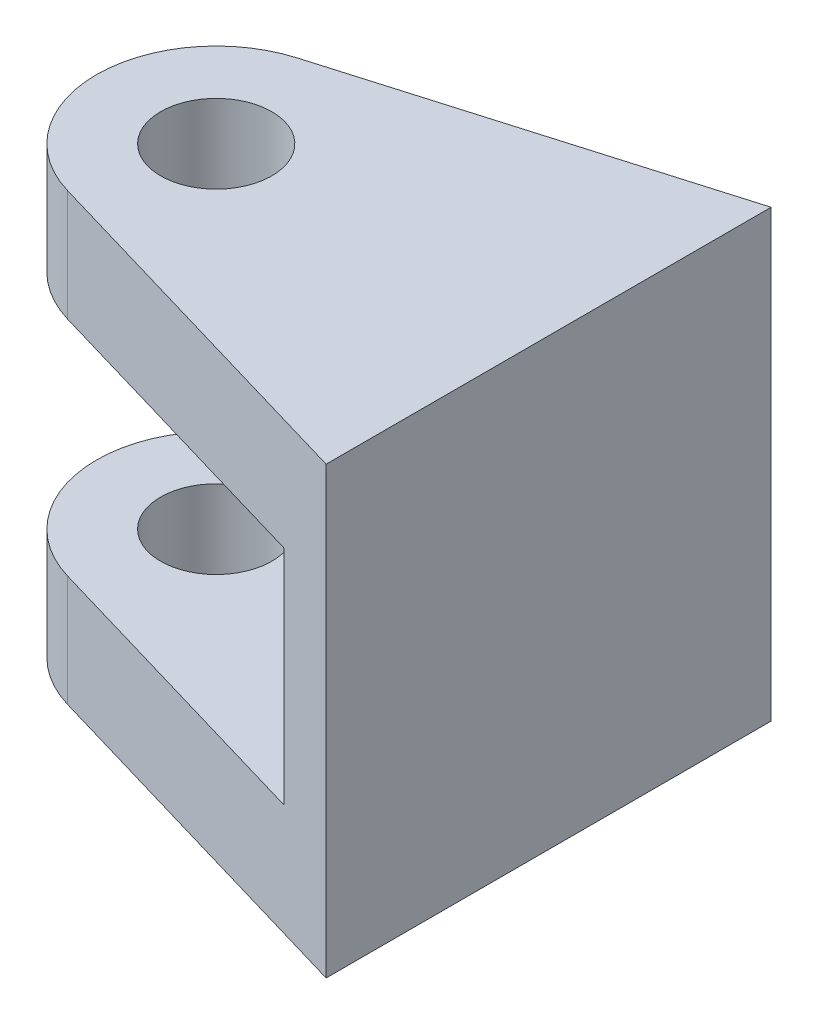
SolidWorks part; units mm, degrees
ref_plane "Front Plane" through (0, 0, 0) normal (0, 0, 1) x (1, 0, 0)
ref_plane "Top Plane" through (0, 0, 0) normal (0, 1, 0) x (1, 0, 0)
ref_plane "Right Plane" through (0, 0, 0) normal (1, 0, 0) x (0, 0, -1)
sketch "Sketch1" plane through (0, 0, 0) normal (0, 1, 0) x (1, 0, 0)
  line L0 (0, 0) -> (0, -40)
  line L1 (0, 0) -> (-32.9168, -9.6735)
  line L2 (0, -40) -> (-32.9168, -30.3265)
  line L3 (0, -20) -> (-54.9892, -20) construction
  arc A1 (-32.9168, -30.3265) -> (-32.9168, -9.6735) centre (-29.8821, -20) cw
  dimension "D1" = 40
extrude "Boss-Extrude1" add sketch "Sketch1" along normal blind 40
ref_plane "Plane1" through (0, 10, 0) normal (0, -1, 0) x (-1, 0, 0)
sketch "Sketch2" plane through (0, 10, 0) normal (0, -1, 0) x (-1, 0, 0)
  line L0 (5.3815, -1.5815) -> (5.3815, -38.4185)
  line L3 (0, 0) -> (0, -40)
  line L4 (0, -40) -> (32.9168, -30.3265)
  line L5 (32.9168, -9.6735) -> (0, 0)
  line L7 (5.3815, -38.4185) -> (32.9168, -30.3265)
  line L8 (32.9168, -9.6735) -> (5.3815, -1.5815)
  arc A1 (32.9168, -30.3265) -> (32.9168, -9.6735) centre (29.8821, -20) ccw
  arc A2 (32.9168, -30.3265) -> (32.9168, -9.6735) centre (29.8821, -20) ccw
  dimension "D1" = 0
extrude "Cut-Extrude1" cut sketch "Sketch2" against normal blind 20
sketch "Sketch3" plane through (0, 10, 0) normal (0, -1, 0) x (-1, 0, 0)
  circle A0 centre (29.8821, -20) radius 5
  dimension "D1" = 10
extrude "Cut-Extrude2" cut sketch "Sketch3" against normal mid plane 140 contours A0
